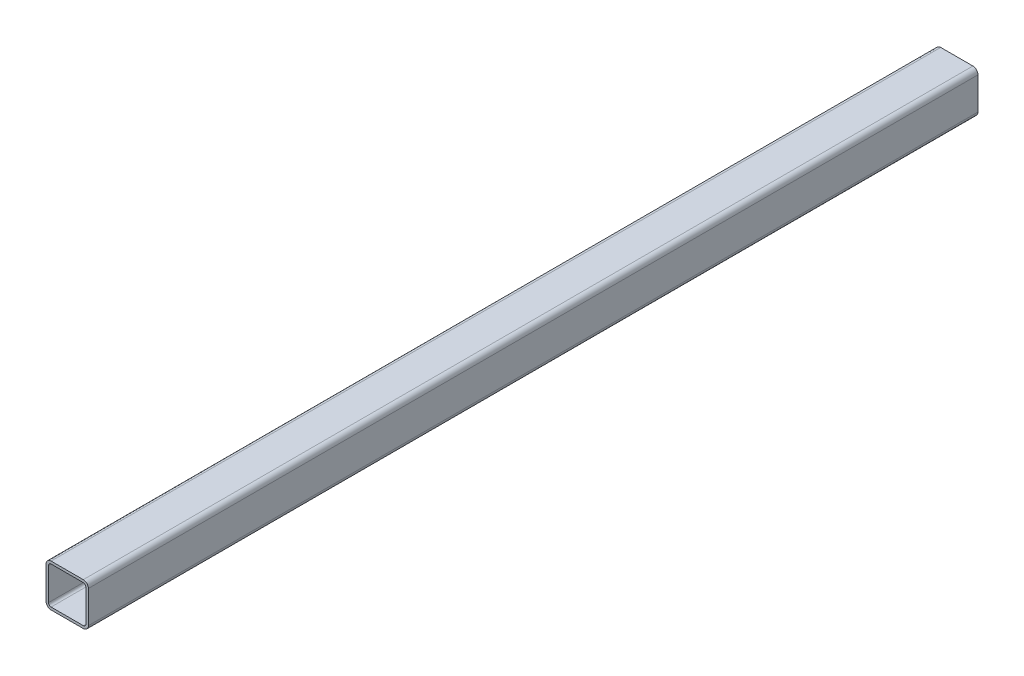
from build123d import *

# Parameters (mm, degrees)
GB_6728_1986_050_X_50_X_3_1_DEPTH = 1050


with BuildPart() as part:
    # Sketch1 → Gb／6728-1986方形空心型钢 050 X 50 X 3(1) (new body)
    with BuildSketch(Plane.YX.offset(-525)):
        with BuildLine():
            Line((-19, -25), (19, -25))
            ThreePointArc((19, -25), (23.242640687, -23.242640687), (25, -19))
            Line((25, -19), (25, 19))
            ThreePointArc((25, 19), (23.242640687, 23.242640687), (19, 25))
            Line((19, 25), (-19, 25))
            ThreePointArc((-19, 25), (-23.242640687, 23.242640687), (-25, 19))
            Line((-25, 19), (-25, -19))
            ThreePointArc((-25, -19), (-23.242640687, -23.242640687), (-19, -25))
        make_face()
        with BuildLine():
            Line((-19, -22), (19, -22))
            ThreePointArc((19, -22), (21.121320344, -21.121320344), (22, -19))
            Line((22, -19), (22, 19))
            ThreePointArc((22, 19), (21.121320344, 21.121320344), (19, 22))
            Line((19, 22), (-19, 22))
            ThreePointArc((-19, 22), (-21.121320344, 21.121320344), (-22, 19))
            Line((-22, 19), (-22, -19))
            ThreePointArc((-22, -19), (-21.121320344, -21.121320344), (-19, -22))
        make_face(mode=Mode.SUBTRACT)
    extrude(amount=GB_6728_1986_050_X_50_X_3_1_DEPTH)


solid = part.part
